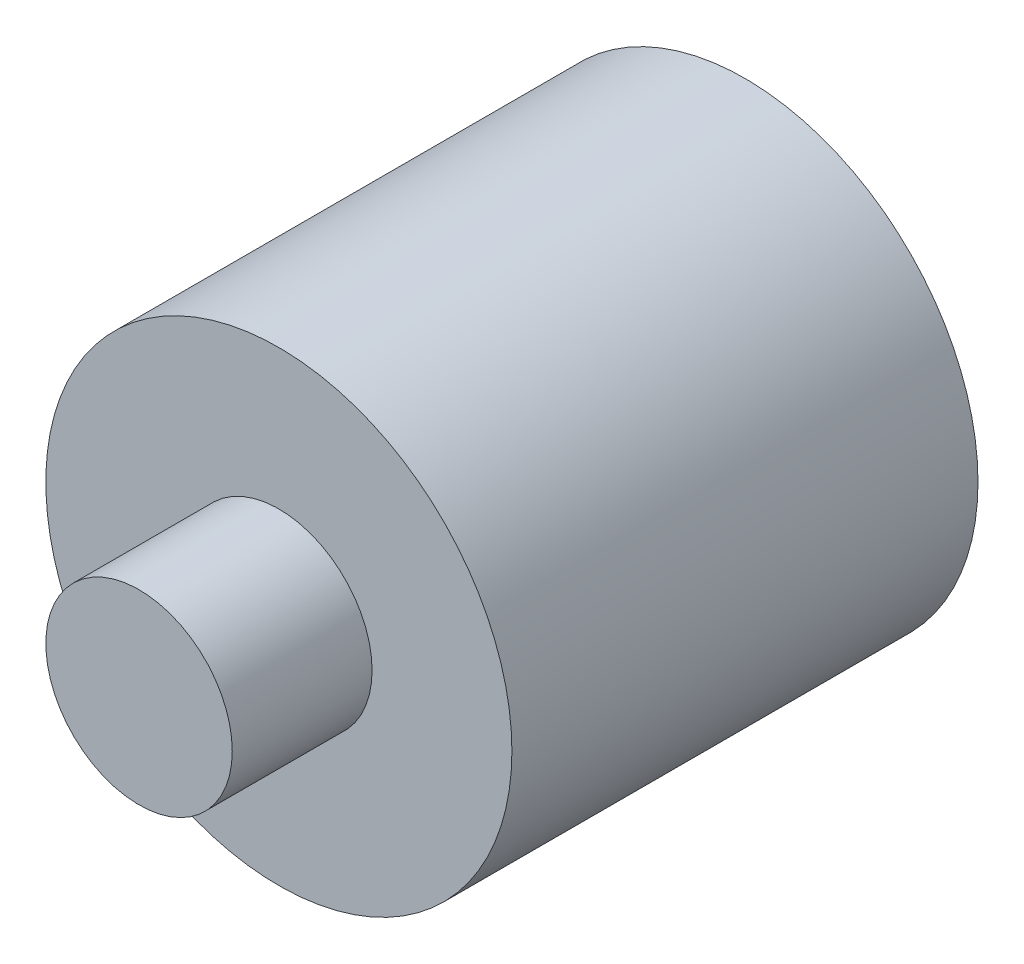
from build123d import *

# Parameters (mm, degrees)
SKETCH1_R           = 2.5
BOSS_EXTRUDE1_DEPTH = 5
SKETCH2_R           = 1
BOSS_EXTRUDE2_DEPTH = 1.5


with BuildPart() as part:
    # Sketch1 → Boss-Extrude1 (new body)
    with BuildSketch(Plane.XY):
        Circle(SKETCH1_R)
    extrude(amount=BOSS_EXTRUDE1_DEPTH)

    # Sketch2 → Boss-Extrude2 (add)
    with BuildSketch(Plane.XY.offset(5)):
        Circle(SKETCH2_R)
    extrude(amount=BOSS_EXTRUDE2_DEPTH)

    # Sketch3 → Cut-Revolve1 (revolve, cut)
    with BuildSketch(Plane(origin=(0, 0, 0), x_dir=(1, 0, 0), z_dir=(0, 1, 0))):
        with BuildLine():
            Line((-2.449489743, 0), (0, 0))
            Line((0, 0), (0, -2))
            ThreePointArc((0, -2), (-1.58113883, -1.436491673), (-2.449489743, 0))
        make_face()
    revolve(axis=Axis((0, 0, 0), (0, 0, -1)), mode=Mode.SUBTRACT)


solid = part.part
